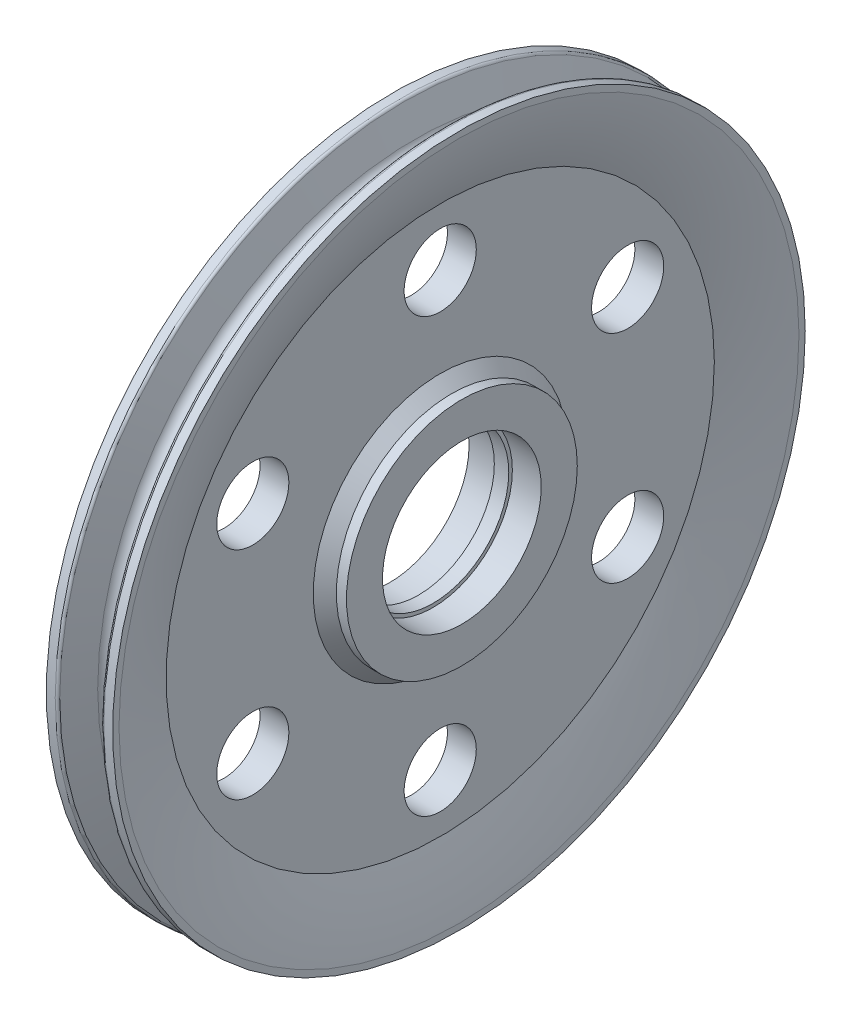
SolidWorks part; units mm, degrees
material "Q235B"
ref_plane "Front Plane" through (0, 0, 0) normal (0, 0, 1) x (1, 0, 0)
ref_plane "Top Plane" through (0, 0, 0) normal (0, 1, 0) x (1, 0, 0)
ref_plane "Right Plane" through (0, 0, 0) normal (1, 0, 0) x (0, 0, -1)
sketch "Sketch1" plane through (0, 0, 0) normal (0, 0, 1) x (1, 0, 0)
  line L0 (0, 0) -> (25, 0) construction
  line L1 (25, 0) -> (25, 80)
  line L2 (25, 80) -> (10, 80)
  line L3 (-23, 235.65) -> (-23, 240)
  line L4 (10, 80) -> (10, 190)
  line L5 (-15.4967, 240) -> (-7.4175, 220.0031)
  line L6 (23, 240) -> (15.4967, 240)
  line L7 (15.4967, 240) -> (7.4175, 220.0031)
  line L8 (0, 0) -> (0, 223) construction
  line L9 (23, 235.65) -> (23, 240)
  line L10 (-23, 240) -> (-15.4967, 240)
  line L11 (-10, 80) -> (-10, 190)
  line L12 (-25, 80) -> (-10, 80)
  line L13 (-25, 0) -> (-25, 80)
  line L14 (25, 0) -> (-25, 0)
  arc A0 (7.4175, 220.0031) -> (-7.4175, 220.0031) centre (0, 223) cw
  arc A1 (10, 190) -> (23, 235.65) centre (-174.4934, 267.2152) ccw
  arc A2 (-10, 190) -> (-23, 235.65) centre (174.4934, 267.2152) cw
  dimension "D1" = 446
  dimension "D4" = 8
  dimension "D7" = 200
  dimension "D2" = 160
  dimension "D3" = 50
  dimension "D5" = 46
  dimension "D6" = 20
  dimension "D8" = 480
  dimension "D9" = 44
  dimension "D10" = 4.35
  dimension "D11" = 50
revolve "Revolve1" add sketch "Sketch1" angle 360 about L14
sketch "Sketch2" plane through (25, 0, 0) normal (1, 0, 0) x (0, 0, -1)
  line L0 (0, 0) -> (0, 150) construction
  line L1 (0, 0) -> (0, 150) construction
  line L2 (0, 0) -> (129.9038, 75) construction
  circle A0 centre (0, 0) radius 52.5
  circle A1 centre (0, 150) radius 25
  circle A2 centre (129.9038, 75) radius 25
  circle A3 centre (129.9038, -75) radius 25
  circle A4 centre (0, -150) radius 25
  circle A5 centre (-129.9038, -75) radius 25
  circle A6 centre (-129.9038, 75) radius 25
  dimension "D1" = 105
  dimension "D2" = 50
  dimension "D5" = 60
  dimension "D6" = 150
  dimension "D4" = 6
extrude "Cut-Extrude1" cut sketch "Sketch2" against normal up to next
sketch "Sketch4" plane through (25, 0, 0) normal (1, 0, 0) x (0, 0, -1)
  circle A1 centre (0, 0) radius 55
  dimension "D1" = 110
extrude "Cut-Extrude2" cut sketch "Sketch4" against normal blind 20
mirror "Mirror1" about plane through (0, 0, 0) normal (1, 0, 0) of "Cut-Extrude2"
chamfer "Chamfer1" distance 8 angle 45 2 edges at (10, 0, -80) (-10, 0, -80)
sketch "Sketch6" plane through (0, 0, 0) normal (0, 0, 1) x (1, 0, 0)
  line L0 (0, 52.5) -> (-35.5212, 114.0245) construction
  line L1 (5, 52.5) -> (-5, 52.5) construction
  line L2 (-7.4175, 220.0031) -> (-7.4175, -220.0031) construction
  line L3 (-21.3294, 89.4437) -> (3.0945, 47.1402)
  line L4 (-21.3294, 89.4437) -> (-19.1644, 90.6937)
  line L5 (3.0945, 47.1402) -> (5.2596, 48.3902)
  line L6 (-19.1644, 90.6937) -> (5.2596, 48.3902)
  dimension "D1" = 30
  dimension "D2" = 2.5
revolve "Cut-Revolve1" cut sketch "Sketch6" angle 360 about L3
cosmetic thread "Cosmetic Thread1" parameters "D1"=10, "D2"=8
fillet "Fillet1" radius 2 2 edges at (-15.4967, 0, -240) (15.4967, 0, -240)
